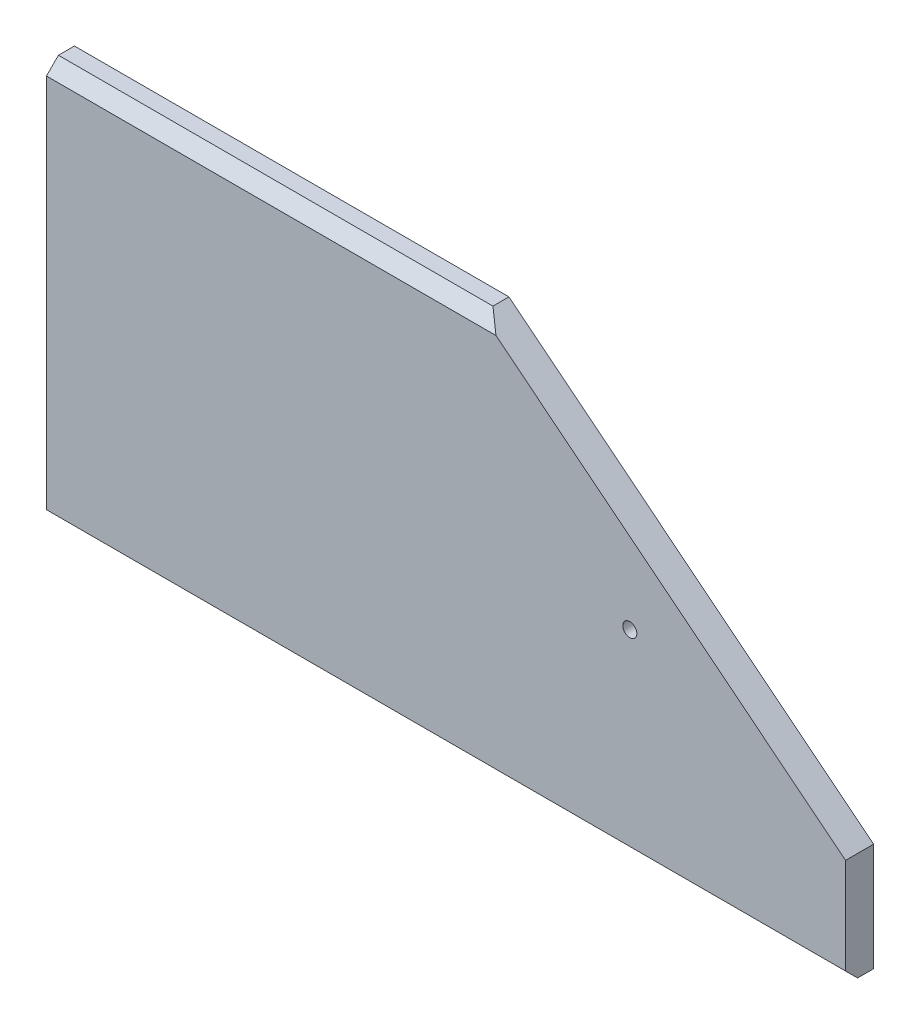
from build123d import *

# Parameters (mm, degrees)
SKETCH1_W           = 1000
SKETCH1_H           = 500
BOSS_EXTRUDE1_DEPTH = 35
M20_TAPPED_HOLE1_D  = 17.5
CHAMFER1_SIZE       = 15
CUT_EXTRUDE3_DEPTH  = 1130.97787589


with BuildPart() as part:
    # Sketch1 → Boss-Extrude1 (new body)
    with BuildSketch(Plane.XY):
        with Locations((-500, -275)):
            Rectangle(SKETCH1_W, SKETCH1_H)
    extrude(amount=-BOSS_EXTRUDE1_DEPTH)

    # M20 Tapped Hole1 (through all)
    with Locations(Plane(origin=(-30, -275, 0), x_dir=(1, 0, 0), z_dir=(0, 0, 1))):
        with Locations((0, 0), (-240, 0)):
            Hole(M20_TAPPED_HOLE1_D / 2)

    # Chamfer1
    chamfer1_edges = [part.edges().sort_by_distance(p)[0] for p in [
        (-500, -525, 0),
        (-500, -25, 0),
    ]]
    chamfer(chamfer1_edges, length=CHAMFER1_SIZE)

    # Sketch9 → Cut-Extrude3 (cut, through all)
    with BuildSketch(Plane.XY):
        Polygon((-500, 10), (0, 10), (0, -390), align=None)
    extrude(amount=-CUT_EXTRUDE3_DEPTH, mode=Mode.SUBTRACT)


solid = part.part
